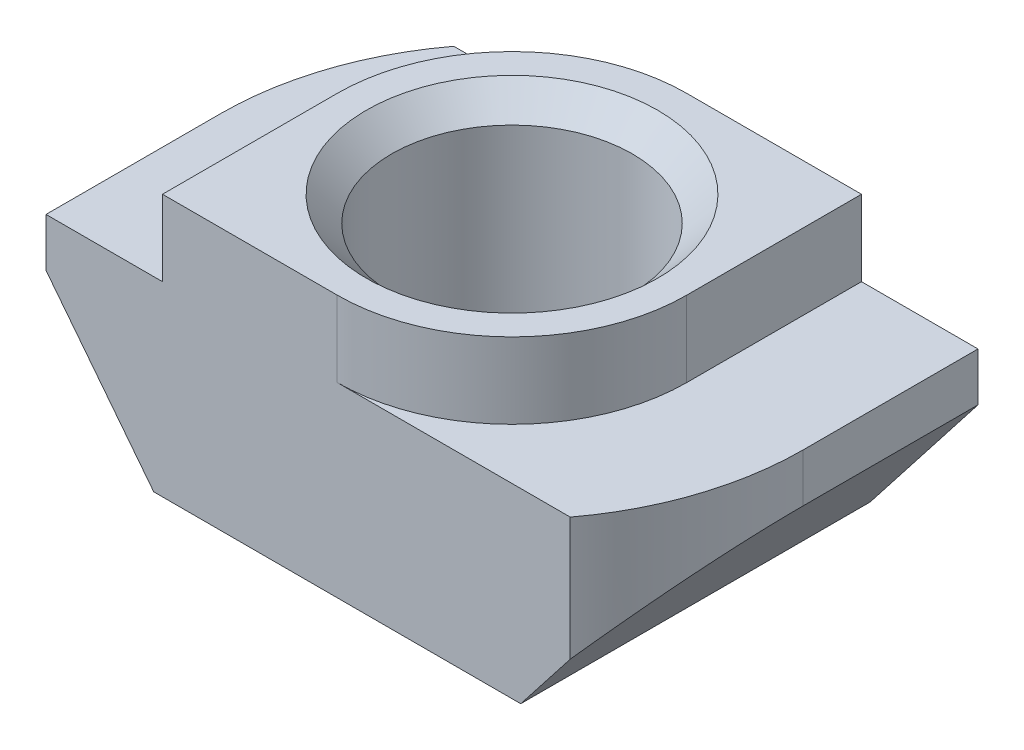
SolidWorks part; units mm, degrees
ref_plane "前视基准面" through (0, 0, 0) normal (0, 0, 1) x (1, 0, 0)
ref_plane "上视基准面" through (0, 0, 0) normal (0, 1, 0) x (1, 0, 0)
ref_plane "右视基准面" through (0, 0, 0) normal (1, 0, 0) x (0, 0, -1)
sketch "草图1" plane through (0, 0, 0) normal (0, 0, 1) x (1, 0, 0)
  line L0 (-5, 2.3679) -> (-3.15, 0)
  line L1 (-3.15, 0) -> (3.15, 0)
  line L2 (3.15, 0) -> (5, 2.3679)
  line L3 (5, 2.3679) -> (5, 3.2)
  line L4 (5, 3.2) -> (3, 3.2)
  line L5 (3, 3.2) -> (3, 4.5)
  line L6 (3, 4.5) -> (-3, 4.5)
  line L7 (-3, 4.5) -> (-3, 3.2)
  line L8 (-3, 3.2) -> (-5, 3.2)
  line L9 (-5, 3.2) -> (-5, 2.3679)
extrude "凸台-拉伸1" add sketch "草图1" along normal blind 6
sketch "草图2" plane through (0, 0, 0) normal (1, 0, 0) x (0, 0, -1)
  line L0 (-3, 0) -> (-5.5, 0)
  line L1 (-5.5, 0) -> (-5.067, 0.433)
  line L2 (-5.067, 0.433) -> (-5.067, 4.067)
  line L3 (-5.067, 4.067) -> (-5.5, 4.5)
  line L4 (-5.5, 4.5) -> (-3, 4.5)
  line L5 (-3, 4.5) -> (-3, 0)
  line L6 (-3, 50) -> (-3, -50) construction
revolve "切除-旋转1" cut sketch "草图2" angle 360 about L6
ref_plane "基准面4" through (0, 4.5, 0) normal (0, 1, 0) x (1, 0, 0)
sketch "草图3" plane through (0, 4.5, 0) normal (0, 1, 0) x (1, 0, 0)
  line L0 (4, -6) -> (5, -6)
  line L1 (5, -6) -> (5, -3)
  arc A0 (5, -3) -> (4, -6) centre (0, -3) cw
extrude "切除-拉伸1" cut sketch "草图3" against normal blind 4.5
ref_plane "基准面5" through (0, 4.5, 0) normal (0, 1, 0) x (1, 0, 0)
sketch "草图4" plane through (0, 4.5, 0) normal (0, 1, 0) x (1, 0, 0)
  line L0 (-4, 0) -> (-5, 0)
  line L1 (-5, 0) -> (-5, -3)
  arc A0 (-5, -3) -> (-4, 0) centre (0, -3) cw
extrude "切除-拉伸2" cut sketch "草图4" against normal blind 4.5
fillet "圆角1" radius 3 2 edges at (3, 3.85, 6) (-3, 3.85, 0)
